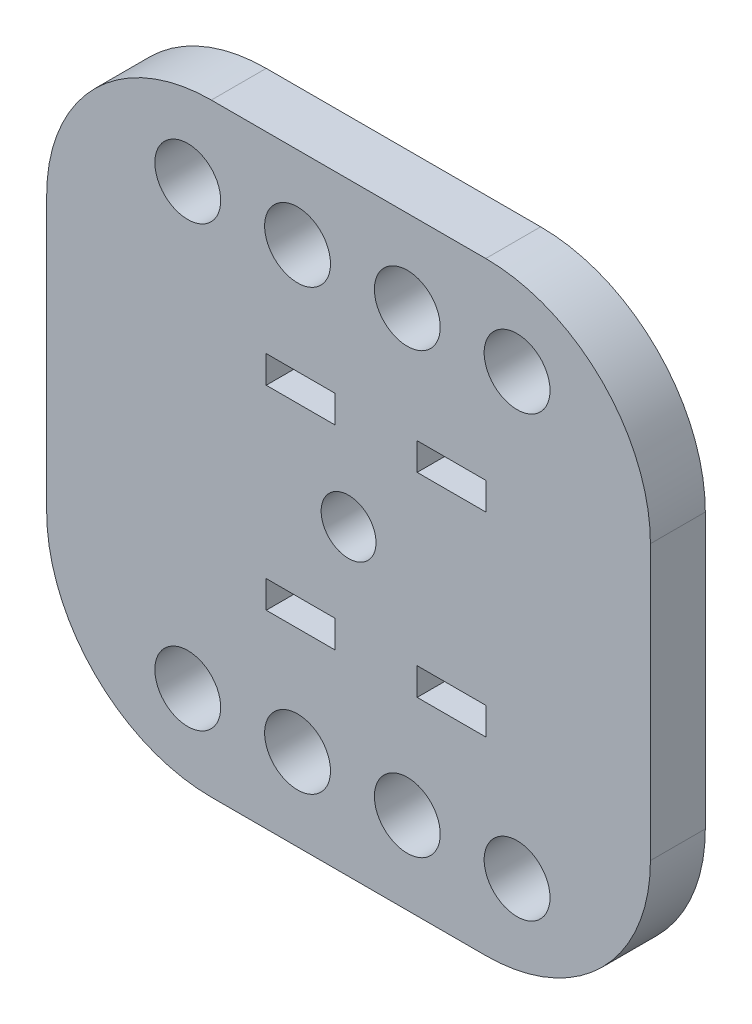
SolidWorks part; units mm, degrees
ref_plane "前视基准面" through (0, 0, 0) normal (0, 0, 1) x (1, 0, 0)
ref_plane "上视基准面" through (0, 0, 0) normal (0, 1, 0) x (1, 0, 0)
ref_plane "右视基准面" through (0, 0, 0) normal (1, 0, 0) x (0, 0, -1)
other "Configuration Table"
sketch "草图1" plane through (0, 0, 0) normal (0, 0, 1) x (1, 0, 0)
  line L0 (-25.4224, 54.8416) -> (24.5776, 54.8416)
  line L1 (-55.4224, 24.8416) -> (-55.4224, -25.1584)
  line L2 (-25.4224, -55.1584) -> (24.5776, -55.1584)
  line L3 (54.5776, 24.8416) -> (54.5776, -25.1584)
  line L4 (12.0776, 14.8416) -> (12.0776, 19.8416)
  line L5 (24.5776, 19.8416) -> (12.0776, 19.8416)
  line L6 (24.5776, 14.8416) -> (24.5776, 19.8416)
  line L7 (24.5776, 14.8416) -> (12.0776, 14.8416)
  line L8 (24.5776, -20.6584) -> (24.5776, -15.6584)
  line L9 (24.5776, -15.6584) -> (12.0776, -15.6584)
  line L10 (12.0776, -20.6584) -> (12.0776, -15.6584)
  line L11 (24.5776, -20.6584) -> (12.0776, -20.6584)
  line L12 (-2.9224, -20.6584) -> (-2.9224, -15.6584)
  line L13 (-15.4224, -20.6584) -> (-15.4224, -15.6584)
  line L14 (-2.9224, -15.6584) -> (-15.4224, -15.6584)
  line L15 (-2.9224, -20.6584) -> (-15.4224, -20.6584)
  line L16 (-2.9224, 19.8416) -> (-15.4224, 19.8416)
  line L17 (-15.4224, 14.8416) -> (-15.4224, 19.8416)
  line L18 (-2.9224, 14.8416) -> (-15.4224, 14.8416)
  line L19 (-2.9224, 14.8416) -> (-2.9224, 19.8416)
  arc A0 (-55.4224, -25.1584) -> (-25.4224, -55.1584) centre (-25.4224, -25.1584) ccw
  arc A1 (24.5776, -55.1584) -> (54.5776, -25.1584) centre (24.5776, -25.1584) ccw
  arc A2 (24.5776, 54.8416) -> (54.5776, 24.8416) centre (24.5776, 24.8416) cw
  arc A3 (-25.4224, 54.8416) -> (-55.4224, 24.8416) centre (-25.4224, 24.8416) ccw
  circle A4 centre (-29.718, 39.8416) radius 6
  circle A5 centre (-9.718, 39.8416) radius 6
  circle A6 centre (10.282, 39.8416) radius 6
  circle A7 centre (30.282, 39.8416) radius 6
  circle A8 centre (30.282, -40.1584) radius 6
  circle A9 centre (10.282, -40.1584) radius 6
  circle A10 centre (-9.718, -40.1584) radius 6
  circle A11 centre (-29.718, -40.1584) radius 6
  dimension "D1" = 30
  dimension "D2" = 12
  dimension "D3" = 20
  dimension "D4" = 20
  dimension "D5" = 20
  dimension "D6" = 30
  dimension "D7" = 15
  dimension "D8" = 15
extrude "凸台-拉伸1" add sketch "草图1" along normal blind 10
sketch "草图2" plane through (0, 0, 0) normal (0, 0, -1) x (-1, 0, 0)
  line L0 (55.4224, 24.8416) -> (55.4224, -25.1584) construction
  circle A0 centre (0.4224, 0) radius 11
  dimension "D1" = 22
  dimension "D2" = 55
extrude "凸台-拉伸2" add sketch "草图2" along normal blind 15
sketch "草图3" plane through (0, 0, -15) normal (0, 0, -1) x (-1, 0, 0)
  circle A0 centre (0.4224, 0) radius 5
extrude "切除-拉伸1" cut sketch "草图3" against normal blind 25
fillet "圆角1" radius 0.5 1 edges at (-5.4224, 0, -15)
fillet "圆角2" radius 0.5 1 edges at (-11.4224, 0, -15)
